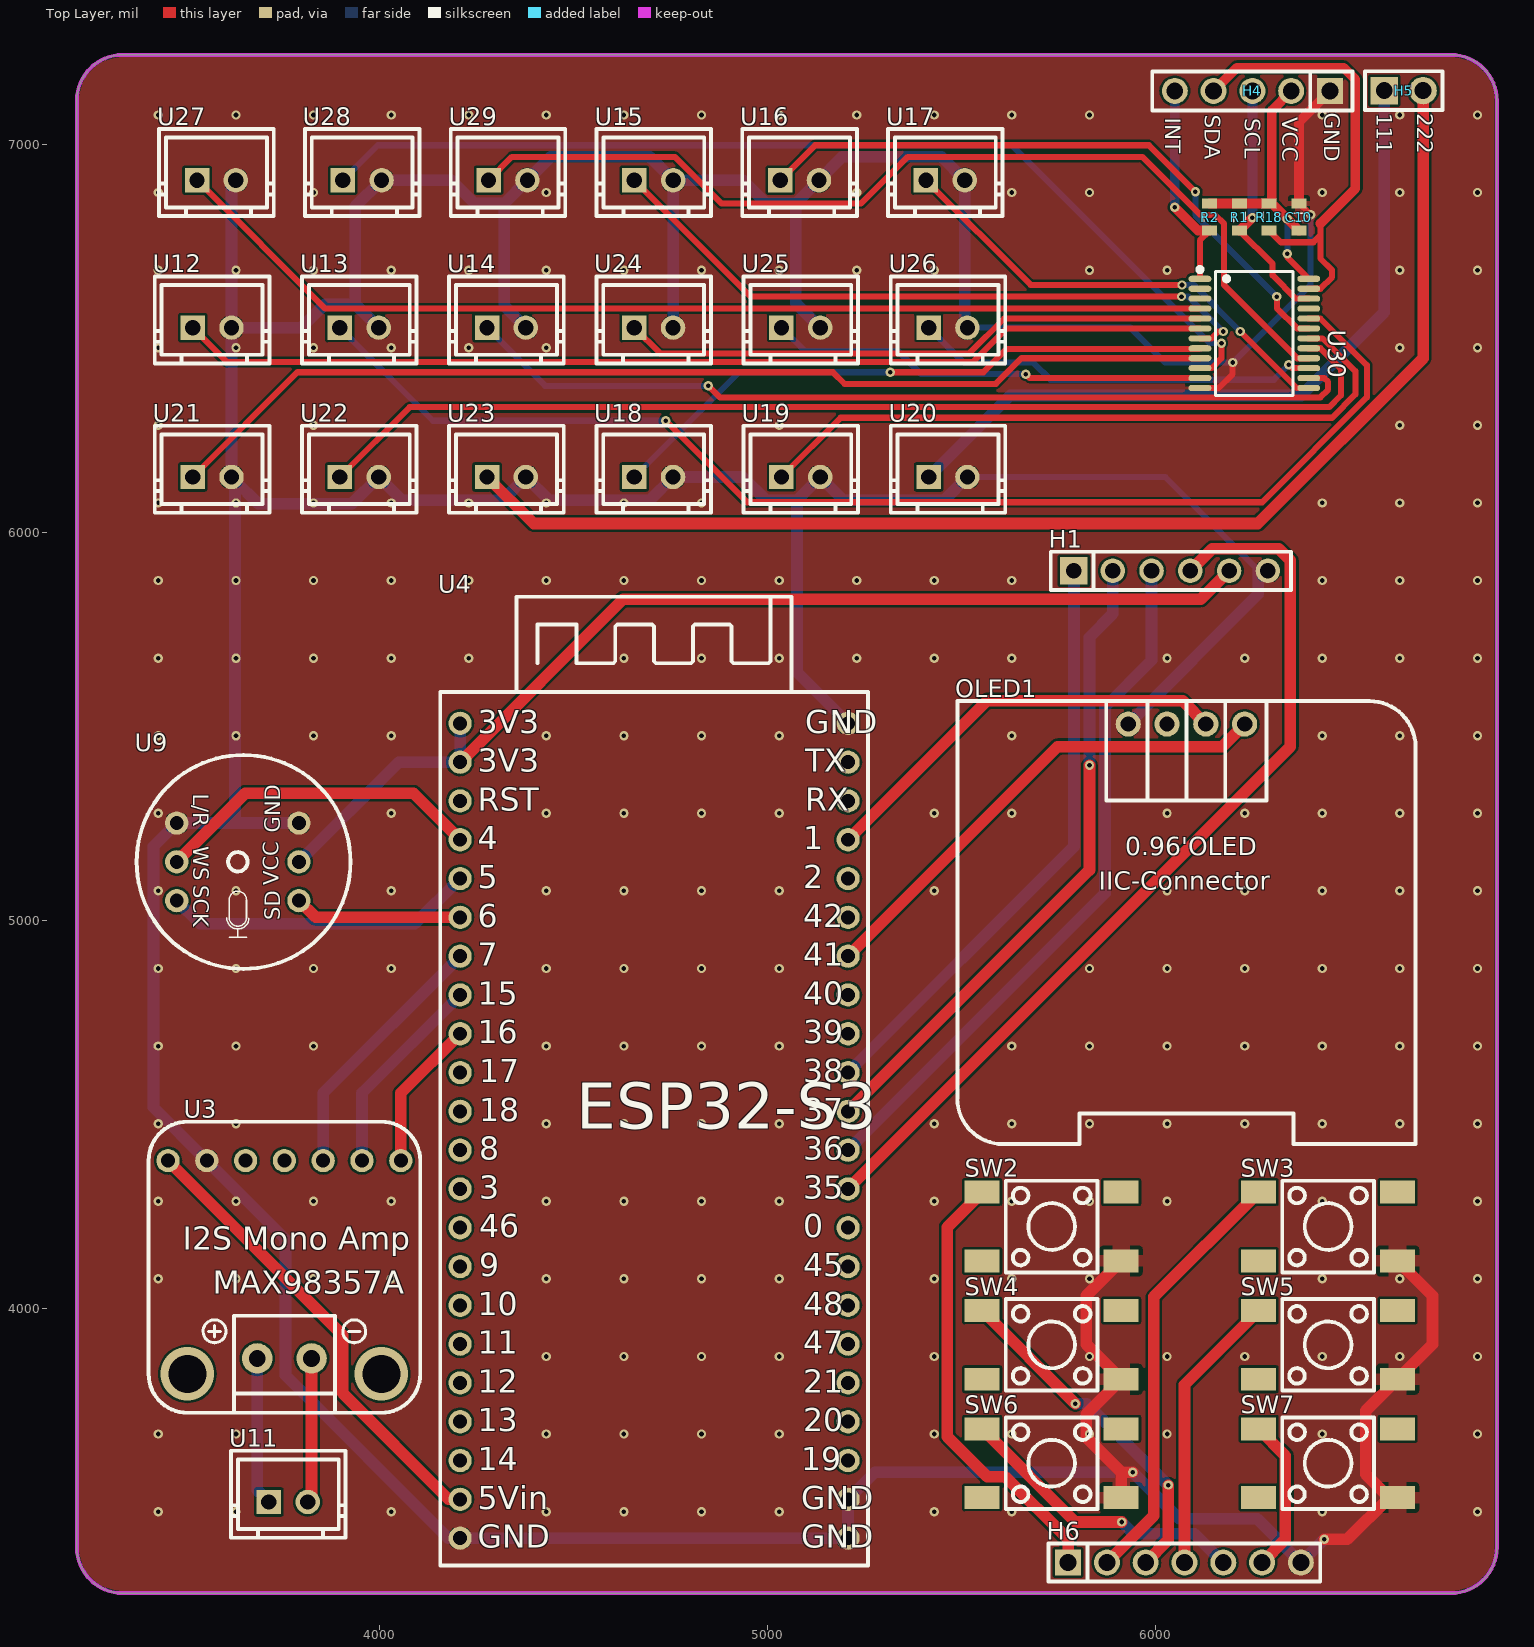
[diagram p0: Top Layer view]
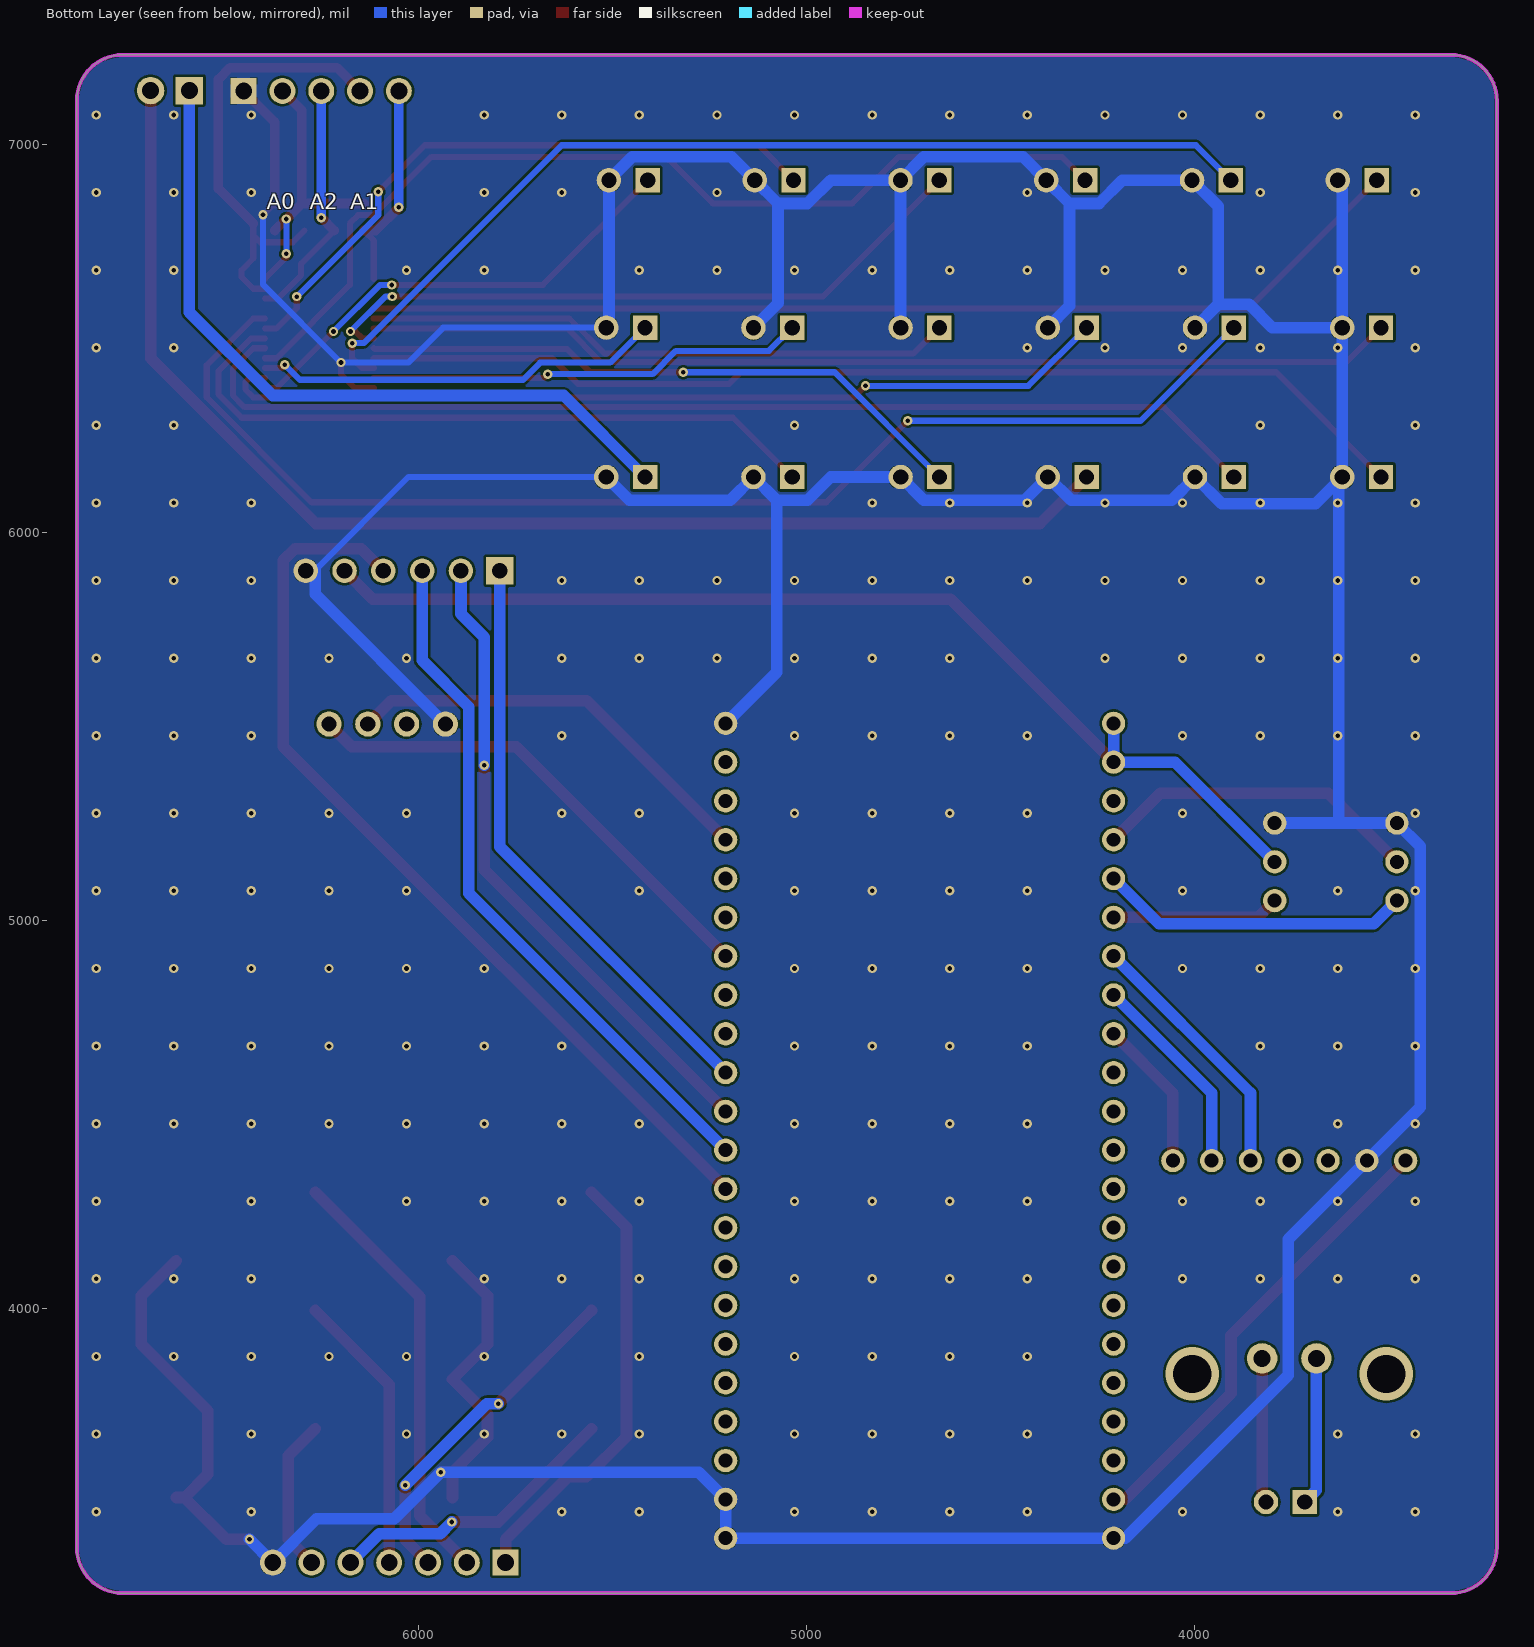
[diagram p1: Bottom Layer view, seen from below]
# Altium PCB MISC49879.pcbdoc
Units mil, origin at the board's own origin, x right, y up, seen from the top; angles counter-clockwise.
Board outline 3660 x 3965 mil, 2 copper layers (Top Layer, Bottom Layer), stack 62.206 mil thick; 38 components, 74 nets, 177 pads, 263 vias.

## Layer stack, top to bottom
Top Solder Mask Layer: solder mask 0.394, Dk 3.3
Top Layer: signal copper 1.379
Dielectric1: surface 59.449, FR4, Dk 4.5
Bottom Layer: signal copper 1.378
Bottom Solder Mask Layer: solder mask 0.394, Dk 3.3

## Board outline
3338.11,7230 ccw(c3338.11,7111.89) 3220,7111.89 3220,3383.11 ccw(c3338.11,3383.11) 3338.11,3265 6761.89,3265 ccw(c6761.89,3383.11) 6880,3383.11 6880,7111.89 ccw(c6761.89,7111.89) 6761.89,7230

## Design rules (kind name [scope] priority, off if disabled: settings)
BoardOutlineClearance Plane_Default_1 [All] p2 off: genericclearance=6 ignorepadtopadclearanceinfootprint=FALSE except(0: Arc-SplitContinuation Track-SplitContinuation SMDPad-SplitContinuation THPad-SplitContinuation Via-SplitContinuation Fill-SplitContinuation Region-SplitContinuation Poly-SplitContinuation Text-SplitContinuation Hole-SplitContinuation; 6: Arc-OutlineEdge Track-OutlineEdge SMDPad-OutlineEdge THPad-OutlineEdge Via-OutlineEdge Fill-OutlineEdge Region-OutlineEdge Poly-OutlineEdge Text-OutlineEdge Hole-OutlineEdge Arc-CutoutEdge Track-CutoutEdge SMDPad-CutoutEdge THPad-CutoutEdge Via-CutoutEdge Fill-CutoutEdge Region-CutoutEdge Poly-CutoutEdge Text-CutoutEdge Hole-CutoutEdge)
BoardOutlineClearance Copper_Default_1 [All] p4 off: genericclearance=6 ignorepadtopadclearanceinfootprint=FALSE except(0: Arc-SplitContinuation Track-SplitContinuation SMDPad-SplitContinuation THPad-SplitContinuation Via-SplitContinuation Fill-SplitContinuation Region-SplitContinuation Poly-SplitContinuation Text-SplitContinuation Hole-SplitContinuation; 6: Arc-OutlineEdge Track-OutlineEdge SMDPad-OutlineEdge THPad-OutlineEdge Via-OutlineEdge Fill-OutlineEdge Region-OutlineEdge Poly-OutlineEdge Text-OutlineEdge Hole-OutlineEdge Arc-CutoutEdge Track-CutoutEdge SMDPad-CutoutEdge THPad-CutoutEdge Via-CutoutEdge Fill-CutoutEdge Region-CutoutEdge Poly-CutoutEdge Text-CutoutEdge Hole-CutoutEdge)
BoardOutlineClearance Copper_gge24019_1 [All] p6 off: genericclearance=6 ignorepadtopadclearanceinfootprint=FALSE except(0: Arc-SplitContinuation Track-SplitContinuation SMDPad-SplitContinuation THPad-SplitContinuation Via-SplitContinuation Fill-SplitContinuation Region-SplitContinuation Poly-SplitContinuation Text-SplitContinuation Hole-SplitContinuation; 6: Arc-OutlineEdge Track-OutlineEdge SMDPad-OutlineEdge THPad-OutlineEdge Via-OutlineEdge Fill-OutlineEdge Region-OutlineEdge Text-OutlineEdge Hole-OutlineEdge Arc-CutoutEdge Track-CutoutEdge SMDPad-CutoutEdge THPad-CutoutEdge Via-CutoutEdge Fill-CutoutEdge Region-CutoutEdge Text-CutoutEdge Hole-CutoutEdge; 10: Poly-OutlineEdge Poly-CutoutEdge)
BoardOutlineClearance Default_1 [All] p8: genericclearance=6 ignorepadtopadclearanceinfootprint=FALSE except(0: Arc-SplitContinuation Track-SplitContinuation SMDPad-SplitContinuation THPad-SplitContinuation Via-SplitContinuation Fill-SplitContinuation Region-SplitContinuation Poly-SplitContinuation Text-SplitContinuation Hole-SplitContinuation; 6: Arc-OutlineEdge Track-OutlineEdge SMDPad-OutlineEdge THPad-OutlineEdge Via-OutlineEdge Fill-OutlineEdge Region-OutlineEdge Poly-OutlineEdge Text-OutlineEdge Hole-OutlineEdge Arc-CutoutEdge Track-CutoutEdge SMDPad-CutoutEdge THPad-CutoutEdge Via-CutoutEdge Fill-CutoutEdge Region-CutoutEdge Poly-CutoutEdge Text-CutoutEdge Hole-CutoutEdge)
Clearance Plane_Default [All] p1 off: gap=6 ignorepadtopadclearanceinfootprint=FALSE
Clearance Copper_Default [All] p3 off: gap=6 ignorepadtopadclearanceinfootprint=FALSE
Clearance Copper_gge24019 [All] p5 off: gap=6 ignorepadtopadclearanceinfootprint=FALSE except(10: Poly-Track Poly-SMDPad Poly-THPad Poly-Via Poly-Fill Poly-Region Poly-Poly Poly-Arc Poly-Text Poly-Hole)
Clearance Default [All] p7: gap=6 ignorepadtopadclearanceinfootprint=FALSE
DiffPairsRouting differentialPair [All] p1: maxlimit=6 minlimit=6 mostfreqgap=6 toplayer_minwidth=5 toplayer_prefwidth=10 toplayer_maxwidth=100 toplayer_mingap=6 toplayer_prefgap=6 toplayer_maxgap=6 bottomlayer_minwidth=5 bottomlayer_prefwidth=10 bottomlayer_maxwidth=100 bottomlayer_mingap=6 bottomlayer_prefgap=6 bottomlayer_maxgap=6 maxuncoupledlength=10
HoleToHoleClearance otherClearance [All] p1: gap=11.8 allowstackedmicrovias=TRUE
Length netLength [All] p1: minlimit=0 maxlimit=0
PasteMaskExpansion Common [All] p1: expansion=0
PlaneConnect Default_4 [All] p1: planeconnectstyle=Relief reliefexpansion=20 reliefentries=4 reliefconductorwidth=0 reliefairgap=10
PolygonConnect gge24019 [All] p1 off: connectstyle=Relief reliefconductorwidth=0 reliefentries=4 polygonreliefangle="90 Angle" airgapwidth=1 via.connectstyle=Relief via.reliefconductorwidth=10 via.reliefentries=4 via.polygonreliefangle="90 Angle" via.airgapwidth=10
PolygonConnect Default_5 [All] p2: connectstyle=Relief reliefconductorwidth=0 reliefentries=4 polygonreliefangle="90 Angle" airgapwidth=1 via.connectstyle=Relief via.reliefconductorwidth=10 via.reliefentries=4 via.polygonreliefangle="90 Angle" via.airgapwidth=10
RoutingVias Default_3 [All] p1: holewidth=12 width=24 viastyle="Through Hole" minholewidth=12 minwidth=24 maxholewidth=2362 maxwidth=3938
SolderMaskExpansion Common_1 [IsVia] p1: expansion=-1000 istentingtop=TRUE
SolderMaskExpansion Common_1 [All] p2: expansion=2 istentingtop=FALSE
Width Default_2 [All] p1: maxlimit=1000 minlimit=10 preferedwidth=30

## Components (designator, comment, footprint, x,y, rotation, side; value= is the part's Value field where it differs from the comment)
C10 "0.1uF" C0603-1 6370,6812 r270 top
H1 "" HDR-TH_6P-P2.54-V-F 6040,5900 r0 top
H4 "KH-2.54PH180-1X5P-L11.5" HDR-TH_5P-P2.54-V-M 6250,7137 r180 top
H5 "" HDR-TH_2P-P2.54-V-M-1 6639.9,7137.78 r0 top
H6 "" HDR-TH_7P-P2.54-V-M 6074.9,3343.84 r0 top
OLED1 "" 0.96OLED_4P 6080,5505 r0 top
R1 "4.7K" R0603-1 6216.67,6812 r90 top
R2 "4.7K" R0603-1 6140,6812 r90 top
R18 "4.7K" R0603-1 6293.33,6812 r90 top
SW2 "KH-6X6X5H-STM" SW-SMD_4P-L6.0-W6.0-P4.50-LS9.0-2 5732.51,4210 r0 top
SW3 "KH-6X6X5H-STM" SW-SMD_4P-L6.0-W6.0-P4.50-LS9.0-2 6445,4210 r0 top
SW4 "KH-6X6X5H-STM" SW-SMD_4P-L6.0-W6.0-P4.50-LS9.0-2 5732.51,3905 r0 top
SW5 "KH-6X6X5H-STM" SW-SMD_4P-L6.0-W6.0-P4.50-LS9.0-2 6445,3905 r0 top
SW6 "KH-6X6X5H-STM" SW-SMD_4P-L6.0-W6.0-P4.50-LS9.0-2 5732.51,3600 r0 top
SW7 "KH-6X6X5H-STM" SW-SMD_4P-L6.0-W6.0-P4.50-LS9.0-2 6445,3600 r0 top
U3 "Adafruit MAX98357 I2S Amp" "MAX98357 I2S AMP MODULE" 3755,4380 r270 top
U4 "NO" ESP32S3 4707.78,4461.89 r0 top
U9 "INMP441" INMP441 3635,5150 r0 top
U11 "_x001F_XH2.54-2P" CONN-TH_2P-P2.54-V 3765,3500 r0 top
U12 "_x001F_XH2.54-2P" CONN-TH_2P-P2.54-V 3568.61,6526.9 r0 top
U13 "_x001F_XH2.54-2P" CONN-TH_2P-P2.54-V 3947.98,6526.9 r0 top
U14 "_x001F_XH2.54-2P" CONN-TH_2P-P2.54-V 4327.34,6526.9 r0 top
U15 "_x001F_XH2.54-2P" CONN-TH_2P-P2.54-V 4707.04,6906.91 r0 top
U16 "_x001F_XH2.54-2P" CONN-TH_2P-P2.54-V 5082.79,6906.91 r0 top
U17 "_x001F_XH2.54-2P" CONN-TH_2P-P2.54-V 5458.54,6906.91 r0 top
U18 "_x001F_XH2.54-2P" CONN-TH_2P-P2.54-V 4706.71,6141.91 r0 top
U19 "_x001F_XH2.54-2P" CONN-TH_2P-P2.54-V 5086.07,6141.91 r0 top
U20 "_x001F_XH2.54-2P" CONN-TH_2P-P2.54-V 5465.44,6141.91 r0 top
U21 "_x001F_XH2.54-2P" CONN-TH_2P-P2.54-V 3568.61,6141.91 r0 top
U22 "_x001F_XH2.54-2P" CONN-TH_2P-P2.54-V 3947.98,6141.91 r0 top
U23 "_x001F_XH2.54-2P" CONN-TH_2P-P2.54-V 4327.34,6141.91 r0 top
U24 "_x001F_XH2.54-2P" CONN-TH_2P-P2.54-V 4706.71,6526.9 r0 top
U25 "_x001F_XH2.54-2P" CONN-TH_2P-P2.54-V 5086.07,6526.9 r0 top
U26 "_x001F_XH2.54-2P" CONN-TH_2P-P2.54-V 5465.44,6526.9 r0 top
U27 "_x001F_XH2.54-2P" CONN-TH_2P-P2.54-V 3579.8,6906.91 r0 top
U28 "_x001F_XH2.54-2P" CONN-TH_2P-P2.54-V 3955.55,6906.91 r0 top
U29 "_x001F_XH2.54-2P" CONN-TH_2P-P2.54-V 4331.3,6906.91 r0 top
U30 "PCF8575TS/1,112" SSOP-24_L8.2-W5.3-P0.65-LS7.8-BL 6255,6512 r270 top

## Footprints (in the part's own frame and the unit in brackets; to place one, negate y for a bottom-side part, rotate by r counter-clockwise, add the part's x,y. Pads: shape width x height; smd on the part's side, far side on the other; paste and mask are expansions set on the pad)
0.96OLED_4P [mm]
  round 1.65 hole 1 copper offset 0,0: 1(-3.81,-0.001) 2(-1.27,0.002) 3(1.27,0.002) 4(3.81,0.002)
  silkscreen extent -15,-27.5 15,1.5
C0603-1 [mil]
  rect 25x38.58 smd paste+0 mask+4: 1(-35,0) 2(35,0)
  silkscreen extent -10,-15 10,16
CONN-TH_2P-P2.54-V [mm]
  rect 1.6x1.6 hole 1: 1(-1.27,0)
  round 1.6 hole 1: 2(1.27,0)
  silkscreen extent -3.75,-2.34 3.75,3.36
ESP32S3 [mil]
  round 60 hole 36: 1(-500,-1055) 2(-500,-955) 3(-500,-855) 4(-500,-755) 5(-500,-655) 6(-500,-555) 7(-500,-455) 8(-500,-355) 9(-500,-255) 10(-500,-155) 11(-500,-55) 12(-500,45) 13(-500,145) 14(-500,245) 15(-500,345) 16(-500,445) 17(-500,545) 18(-500,645) 19(-500,745) 20(-500,845) 21(-500,945) 22(-500,1045) 23(500,-1055) 24(500,-955) 25(500,-855) 26(500,-755) 27(500,-655) 28(500,-555) 29(500,-455) 30(500,-355) 31(500,-255) 32(500,-155) 33(500,-55) 34(500,45) 35(500,145) 36(500,245) 37(500,345) 38(500,445) 39(500,545) 40(500,645) 41(500,745) 42(500,845) 43(500,945) 44(500,1045)
  silkscreen extent -551,-1126 551,1371
HDR-TH_2P-P2.54-V-M-1 [mm]
  rect 1.8x1.8 hole 1.1: 1(-1.27,0)
  round 1.8 hole 1.1: 2(1.27,0)
  silkscreen extent -2.54,-1.27 2.54,1.27
HDR-TH_5P-P2.54-V-M [mm]
  rect 1.7x1.7 hole 1.1: 1(-5.08,0)
  round 1.7 hole 1.1: 2(-2.54,0) 3(0,0) 4(2.54,0) 5(5.08,0)
  silkscreen extent -6.56,-1.27 6.56,1.27
HDR-TH_6P-P2.54-V-F [mm]
  rect 1.8x1.8 hole 1.02: 1(-6.35,0)
  round 1.6 hole 1.02: 2(-3.81,0) 3(-1.27,0) 4(1.27,0) 5(3.81,0) 6(6.35,0)
  silkscreen extent -7.87,-1.25 7.87,1.25
HDR-TH_7P-P2.54-V-M [mm]
  rect 1.7x1.7 hole 1.1: 1(-7.62,0)
  round 1.7 hole 1.1: 2(-5.08,0) 3(-2.54,0) 4(0,0) 5(2.54,0) 6(5.08,0) 7(7.62,0)
  silkscreen extent -8.89,-1.25 8.89,1.25
INMP441 [mil]
  round 60 hole 36: 1(157.49,100) 2(157.49,0) 3(157.49,-100) 4(-157.47,100) 5(-157.47,0) 6(-157.47,-100)
  silkscreen extent -261,-276 290,275
"MAX98357 I2S AMP MODULE" [mil]
  round 60 hole 36: 1(0,300) 2(0,200) 3(0,100) 4(0,0) 5(0,-100) 6(0,-200) 7(0,-300)
  round 78.74 hole 43.31 paste+0 mask+4: 8(510,-70) 9(510,70)
  silkscreen extent -100,-350 650,350
R0603-1 [mil]
  rect 25x38.58 smd paste+0 mask+4: 1(-35,0) 2(35,0)
  silkscreen extent -13,-15 12,15
SSOP-24_L8.2-W5.3-P0.65-LS7.8-BL [mm]
  oval 0.4x1.5 smd: 1(-3.575,-3.562) 2(-2.925,-3.562) 3(-2.275,-3.562) 4(-1.625,-3.562) 5(-0.975,-3.562) 6(-0.325,-3.562) 7(0.325,-3.562) 8(0.975,-3.562) 9(1.625,-3.562) 10(2.275,-3.562) 11(2.925,-3.562) 12(3.575,-3.562) 13(3.575,3.562) 14(2.925,3.562) 15(2.275,3.562) 16(1.625,3.562) 17(0.975,3.562) 18(0.325,3.562) 19(-0.325,3.562) 20(-0.975,3.562) 21(-1.625,3.562) 22(-2.275,3.562) 23(-2.925,3.562) 24(-3.575,3.562)
  silkscreen extent -4.33,-3.71 4.06,2.54
SW-SMD_4P-L6.0-W6.0-P4.50-LS9.0-2 [mm]
  rect 2.3x1.5 smd: 1(-4.55,2.25) 2(4.55,2.25) 3(-4.55,-2.25) 4(4.55,-2.25)
  silkscreen extent -3,-3 3,3

## Via types
v1: diameter 24, hole 12, Top Layer to Bottom Layer, 261 vias
v2: diameter 137.8, hole 98.4, Top Layer to Bottom Layer, 2 vias

## Nets (pads, with @x,y where several pads share a name; then routed paths per layer and width w, separated by ;. In a path a pad name is that pad's centre, name@x,y a point inside that pad or via, vN(x,y) a via of type N, cw(c..) or ccw(c..) an arc to the next point about the centre after c; other vN are vias at no path point)
0: U4.31
1: OLED1.3 U4.41 | length 1095.4
  Top Layer w30: U4.41 5565.94,5565.05 6070,5565.05 OLED1.3@6130,5505.05
2: U4.40
3: U4.10
3.3V: H1.5 U4.21 U4.22 U9.2 | length 2808.2
  Top Layer w30: U4.21 4627.78,5826.89 6116.89,5826.89 H1.5
  Bottom Layer w30: U9.2 4049.37,5406.89 U4.21 U4.22
4: U4.19 U9.5 | length 853.2
  Top Layer w30: U9.5 3654.41,5326.89 4087.78,5326.89 U4.19
5: U4.18 U9.6 | length 803.5
  Bottom Layer w30: U9.6 3537.52,4990 4090.89,4990 U4.18
5V-VIN: U3.7 U4.2 | length 1202.3
  Top Layer w30: U3.7 3905,3930 3905,3780 4178.11,3506.89 U4.2
6: U4.17 U9.3 | length 433.2
  Top Layer w30: U9.3 3835.59,5006.89 U4.17
7: U3.3 U4.16 | length 673
  Bottom Layer w30: U3.3 3855,4554.11 U4.16
8: U4.11
9: U4.8
10: U4.7
11: U4.6
12: U4.5
13: U4.4
14: U4.3
15: U3.2 U4.15 | length 531.6
  Bottom Layer w30: U3.2 3955,4554.11 U4.15
16: U3.1 U4.14 | length 390.2
  Top Layer w30: U3.1 4055,4554.11 U4.14
17: U4.13
18: U4.12
19: U4.25
20: U4.26
21: U4.27
35: H1.4 U4.32 | length 2386
  Top Layer w30: U4.32 6347.78,5446.89 6347.78,5926.89 6317.78,5956.89 6146.89,5956.89 H1.4
36: H1.3 U4.33 | length 1817.1
  Bottom Layer w30: U4.33 5870,5069.11 5870,5549.11 5990,5669.11 H1.3
37: H1.2 U4.34 | length 1675.7
  Top Layer w30: U4.34 5830,5129.11 v1(5830,5399.11)
  Bottom Layer w30: v1(5830,5399.11) 5830,5729.11 5890,5789.11 H1.2
38: H1.1 U4.35 | length 1534.3
  Bottom Layer w30: U4.35 5790,5189.11 H1.1
39: U4.36
40: U4.37
41: OLED1.4 U4.38 | length 1270
  Top Layer w30: U4.38 5747.78,5446.89 6171.84,5446.89 OLED1.4@6230,5505.05
42: U4.39
45: U4.30
46: U4.9
47: U4.28
48: U4.29
111: H5.1 U20.1 | length 1921.7
  Bottom Layer w30: U20.1 5625.44,6351.91 6375.44,6351.91 6589.9,6566.37 H5.1
222: H5.2 U23.1 | length 3328.7
  Top Layer w30: U23.1 4397.34,6021.91 6264.03,6021.91 6689.9,6447.78 H5.2
$1N6791: H6.1 SW2.1 | length 1148.5
  Top Layer w30: SW2.1 5463.38,4208.59 5463.38,3668.59 5566.6,3565.36 5613.38,3565.36 5774.9,3403.84 H6.1
$1N6796: H6.2 SW3.1 | length 1116.7
  Top Layer w30: H6.2 5995.87,3464.81 5995.87,4028.59 SW3.1
$1N6804: H6.3 SW4.1 | length 890.4
  Top Layer w30: SW4.1 v1(5793.38,3753.59) ; H6.3 6033.38,3402.32 v1(6033.38,3543.59)
  Bottom Layer w30: v1(5793.38,3753.59) 5823.38,3753.59 v1(6033.38,3543.59)
$1N6814: H6.4 SW5.1 | length 728.8
  Top Layer w30: H6.4 6074.9,3802.61 SW5.1
$1N6821: H6.5 SW6.1 | length 764.3
  Top Layer w30: SW6.1 5793.38,3448.59 v1(5913.38,3448.59)
  Bottom Layer w30: v1(5913.38,3448.59) 5943.38,3418.59 6100.15,3418.59 H6.5
$1N6831: H6.6 SW7.1 | length 398.2
  Top Layer w30: SW7.1 6334.9,3619.56 6334.9,3403.84 H6.6
+5V: OLED1.2
A0: U30.21
A1: U30.2
A2: U30.3
GND: C10.1 H1.6 H4.1 H6.7 OLED1.1 SW2.4 SW3.4 SW4.4 SW5.4 SW6.4 SW7.4 U3.6 U4.1 U4.23 U4.24 U4.44 U9.1 U9.4 U12.2 U13.2 U14.2 U15.2 U16.2 U17.2 U18.2 U19.2 U20.2 U21.2 U22.2 U23.2 U24.2 U25.2 U26.2 U27.2 U28.2 U29.2 U30.12 | length 18226.5
  Top Layer w15.75: U30.12 6163.46,6371.25 6199.11,6406.9 v1(6199.11,6436.9) ; C10.1 v1(6400,6817.79)
  Top Layer w25: C10.1 6370,7057 H4.1
  Top Layer w30: SW6.4 5911.64,3576.41 ; SW2.4 5821.64,4031.41 5821.64,3906.41 SW4.4 5821.64,3726.41 5821.64,3666.41 5911.64,3576.41 ; v1(5941.64,3576.41) 5911.64,3576.41 ; v1(6434.9,3403.84) 6494.9,3403.84 SW7.4@6602.48,3511.41 ; SW7.4 SW7.4@6602.48,3511.41 ; SW3.4 6714.13,4031.41 6714.13,3906.41 SW5.4 6542.48,3734.76 6542.48,3571.41 SW7.4@6602.48,3511.41
  Bottom Layer w15.75: U20.2 6025.44,6141.91 6265.44,5901.91 H1.6 ; U26.2 5935.44,6526.9 6025.44,6436.9 v1(6199.11,6436.9) 6400,6637.79 v1(6400,6817.79)
  Bottom Layer w30: U27.2 3618.61,6895.72 U12.2 ; U9.1 3627.52,5250 ; U13.2 3937.98,6586.9 ; U14.2 4321.3,6582.94 4321.3,6846.91 ; U24.2 4757.04,6527.24 U15.2 ; U25.2 5072.79,6590.18 5072.79,6846.91 ; U4.44 5076.07,5638.6 5076.07,6081.91 ; U20.2 5455.44,6081.91 5196.07,6081.91 U19.2 5076.07,6081.91 ; U26.2 5508.54,6533.8 U17.2 5448.54,6966.91 5192.79,6966.91 U16.2 5072.79,6846.91 ; OLED1.1 6265.44,5840.39 H1.6@6265.44,5901.91 ; v1(6434.9,3403.84) H6.7 6262.32,3456.41 6061.64,3456.41 v1(5941.64,3576.41) 5277.3,3576.41 U4.24 U4.23 U4.1 4177.78,3406.89 3757.78,3826.89 3757.78,4177.22 U3.6 3417.52,4517.48 3417.52,5190 U9.4 3627.52,5250 ; U12.2 U21.2 U21.2@3627.52,6133 ; U12.2 3798.61,6526.9 3858.61,6586.9 3937.98,6586.9 ; 3627.52,5250 U21.2@3627.52,6133 ; U21.2@3627.52,6133 3687.52,6073 3929.07,6073 U22.2 4057.98,6081.91 4317.34,6081.91 U23.2 4437.34,6081.91 4696.71,6081.91 U18.2 4936.71,6141.91 4996.71,6081.91 5076.07,6081.91 ; 3937.98,6586.9 3937.98,6839.33 U28.2 4185.55,6906.91 4245.55,6846.91 4321.3,6846.91 ; 4321.3,6846.91 U29.2 4441.3,6966.91 4697.04,6966.91 U15.2 ; U15.2 4937.04,6906.91 4997.04,6846.91 5072.79,6846.91
  other v1: 3430.1,3475.1 3630.1,3475.1 4030.1,3475.1 4430.1,3475.1 4630.1,3475.1 4830.1,3475.1 5030.1,3475.1 5430.1,3475.1 5630.1,3475.1 6430.1,3475.1 6830.1,3475.1 3430.1,3675.1 3630.1,3675.1 4430.1,3675.1 4630.1,3675.1 4830.1,3675.1 5030.1,3675.1 5430.1,3675.1 5630.1,3675.1 5830.1,3675.1 6030.1,3675.1 6430.1,3675.1 6830.1,3675.1 4430.1,3875.1 4630.1,3875.1 4830.1,3875.1 5030.1,3875.1 5430.1,3875.1 5830.1,3875.1 6030.1,3875.1 6230.1,3875.1 6430.1,3875.1 6630.1,3875.1 6830.1,3875.1 3430.1,4075.1 3630.1,4075.1 3830.1,4075.1 4030.1,4075.1 4430.1,4075.1 4630.1,4075.1 4830.1,4075.1 5030.1,4075.1 5430.1,4075.1 5630.1,4075.1 5830.1,4075.1 6430.1,4075.1 6630.1,4075.1 6830.1,4075.1 3430.1,4275.1 3630.1,4275.1 3830.1,4275.1 4030.1,4275.1 4430.1,4275.1 4630.1,4275.1 4830.1,4275.1 5030.1,4275.1 5430.1,4275.1 5630.1,4275.1 5830.1,4275.1 6030.1,4275.1 6430.1,4275.1 6830.1,4275.1 3430.1,4475.1 3630.1,4475.1 4430.1,4475.1 4630.1,4475.1 4830.1,4475.1 5030.1,4475.1 5430.1,4475.1 5630.1,4475.1 5830.1,4475.1 6030.1,4475.1 6230.1,4475.1 6430.1,4475.1 6630.1,4475.1 6830.1,4475.1 3430.1,4675.1 3630.1,4675.1 3830.1,4675.1 4430.1,4675.1 4630.1,4675.1 4830.1,4675.1 5030.1,4675.1 5630.1,4675.1 5830.1,4675.1 6030.1,4675.1 6230.1,4675.1 6430.1,4675.1 6630.1,4675.1 6830.1,4675.1 3430.1,4875.1 3630.1,4875.1 3830.1,4875.1 4030.1,4875.1 4430.1,4875.1 4630.1,4875.1 4830.1,4875.1 5030.1,4875.1 5830.1,4875.1 6030.1,4875.1 6230.1,4875.1 6430.1,4875.1 6630.1,4875.1 6830.1,4875.1 3430.1,5075.1 3630.1,5075.1 4030.1,5075.1 4430.1,5075.1 4630.1,5075.1 4830.1,5075.1 5030.1,5075.1 5430.1,5075.1 6030.1,5075.1 6230.1,5075.1 6430.1,5075.1 6630.1,5075.1 6830.1,5075.1 3430.1,5275.1 4030.1,5275.1 4430.1,5275.1 4630.1,5275.1 4830.1,5275.1 5030.1,5275.1 5430.1,5275.1 5630.1,5275.1 6030.1,5275.1 6230.1,5275.1 6430.1,5275.1 6630.1,5275.1 6830.1,5275.1 3430.1,5475.1 3630.1,5475.1 3830.1,5475.1 4030.1,5475.1 4430.1,5475.1 4630.1,5475.1 4830.1,5475.1 5030.1,5475.1 5630.1,5475.1 6430.1,5475.1 6630.1,5475.1 6830.1,5475.1 3430.1,5675.1 3630.1,5675.1 3830.1,5675.1 4030.1,5675.1 4230.1,5675.1 4630.1,5675.1 4830.1,5675.1 5030.1,5675.1 5230.1,5675.1 5430.1,5675.1 5630.1,5675.1 6030.1,5675.1 6230.1,5675.1 6430.1,5675.1 6630.1,5675.1 6830.1,5675.1 3430.1,5875.1 3630.1,5875.1 3830.1,5875.1 4030.1,5875.1 4230.1,5875.1 4430.1,5875.1 4630.1,5875.1 4830.1,5875.1 5030.1,5875.1 5230.1,5875.1 5430.1,5875.1 5630.1,5875.1 6430.1,5875.1 6630.1,5875.1 6830.1,5875.1 3430.1,6075.1 3630.1,6075.1 3830.1,6075.1 4030.1,6075.1 4230.1,6075.1 4430.1,6075.1 4630.1,6075.1 4830.1,6075.1 6430.1,6075.1 6630.1,6075.1 6830.1,6075.1 3430.1,6275.1 3830.1,6275.1 5030.1,6275.1 6630.1,6275.1 6830.1,6275.1 3430.1,6475.1 3630.1,6475.1 3830.1,6475.1 4030.1,6475.1 4230.1,6475.1 4430.1,6475.1 6630.1,6475.1 6830.1,6475.1 3430.1,6675.1 3630.1,6675.1 3830.1,6675.1 4030.1,6675.1 4230.1,6675.1 4430.1,6675.1 4630.1,6675.1 4830.1,6675.1 5030.1,6675.1 5230.1,6675.1 5430.1,6675.1 5830.1,6675.1 6030.1,6675.1 6630.1,6675.1 6830.1,6675.1 3430.1,6875.1 3830.1,6875.1 4430.1,6875.1 5230.1,6875.1 5630.1,6875.1 5830.1,6875.1 6430.1,6875.1 6630.1,6875.1 6830.1,6875.1 3430.1,7075.1 3630.1,7075.1 3830.1,7075.1 4030.1,7075.1 4230.1,7075.1 4430.1,7075.1 4630.1,7075.1 4830.1,7075.1 5030.1,7075.1 5230.1,7075.1 5430.1,7075.1 5630.1,7075.1 5830.1,7075.1 6430.1,7075.1 6630.1,7075.1 6830.1,7075.1
INT: H4.5 R2.1 U30.1 | length 549.6
  Top Layer w15.75: U30.1 6114.76,6751.76 R2.1
  Top Layer w25: v1(6050,6837) 6110,6777 R2.1
  Bottom Layer w25: v1(6050,6837) H4.5
P00: U27.1 U30.4 | length 2722
  Top Layer w15.75: U27.1 3860.73,6575.98 U30.4
P01: U24.1 U30.5 | length 1522.9
  Top Layer w15.75: U24.1 4723.22,6460.39 5520.2,6460.39 5610.2,6550.39 U30.5
P02: U12.1 U30.6 | length 2669.1
  Top Layer w15.75: U12.1 3607.72,6437.79 5529.5,6437.79 5616.5,6524.79 U30.6
P03: U15.1 U30.7 | length 1746.6
  Top Layer w15.75: U15.1 4957.04,6606.91 v1(6067.04,6606.91) ; U30.7 6144.76,6499.2 6162.47,6516.91 v1(6174.76,6516.91)
  Bottom Layer w15.75: v1(6067.04,6606.91) 6084.76,6606.91 v1(6174.76,6516.91)
P04: U18.1 U30.8 | length 1595.4
  Top Layer w15.75: v1(5316.71,6411.91) 5556.71,6411.91 5616.71,6471.91 6113.06,6471.91 U30.8
  Bottom Layer w15.75: U18.1 4926.71,6411.91 v1(5316.71,6411.91)
P05: U21.1 U30.9 | length 2747.8
  Top Layer w15.75: U21.1 3788.61,6411.91 5168.61,6411.91 5198.61,6381.91 5588.61,6381.91 5654.72,6448.02 U30.9
P06: U28.1 U30.10 | length 2618.3
  Top Layer w15.75: U30.10 6144.76,6422.43 6170.28,6447.95 v1(6170.28,6486.91)
  Bottom Layer w15.75: U28.1 3995.55,6996.91 5630.28,6996.91 6140.28,6486.91 v1(6170.28,6486.91)
P07: U25.1 U30.11 | length 1132.6
  Top Layer w15.75: v1(5666.07,6406.9) 5676.13,6396.84 U30.11
  Bottom Layer w15.75: U25.1 5096.07,6466.9 5336.07,6466.9 5396.07,6406.9 v1(5666.07,6406.9)
P08: U17.1 U30.13 | length 1208.6
  Top Layer w15.75: U17.1 5678.54,6636.91 v1(6068.54,6636.91) ; v1(6218.54,6516.91) 6364.2,6371.25 U30.13
  Bottom Layer w15.75: v1(6068.54,6636.91) 6098.54,6636.91 v1(6218.54,6516.91)
P09: U14.1 U30.14 | length 2324.9
  Top Layer w15.75: v1(4847.34,6376.9) 4877.34,6346.9 6425.24,6346.9 6445.27,6366.93 6445.27,6386.87 6435.3,6396.84 U30.14
  Bottom Layer w15.75: U14.1 4427.34,6376.9 v1(4847.34,6376.9)
P10: U26.1 U30.15 | length 1055.1
  Top Layer w15.75: v1(6343.91,6431.1) 6352.59,6422.43 U30.15
  Bottom Layer w15.75: U26.1 5505.44,6436.9 5685.44,6436.9 5729.91,6392.43 6305.24,6392.43 v1(6343.91,6431.1)
P11: U29.1 U30.16 | length 2546
  Top Layer w15.75: U29.1 4341.3,6966.91 4761.3,6966.91 4881.3,6846.91 5241.3,6846.91 5361.3,6966.91 5966.35,6966.91 6116.35,6816.91 6154.84,6816.91 6176.35,6795.4 6176.35,6636.91 6365.24,6448.02 U30.16
P12: U22.1 U30.17 | length 2840.5
  Top Layer w15.75: U22.1 4077.98,6321.91 6447.98,6321.91 6477.98,6351.91 6477.98,6420.87 6425.24,6473.61 U30.17
P13: U19.1 U30.18 | length 1782.3
  Top Layer w15.75: U19.1 5188.78,6294.62 6455.24,6294.62 6515.24,6354.62 6515.24,6414.62 6430.66,6499.2 U30.18
P14: U16.1 U30.19 | length 1648
  Top Layer w15.75: U16.1 5122.79,6996.91 5983.12,6996.91 v1(6103.12,6876.91) ; v1(6313.12,6606.91) 6313.12,6576.91 6365.24,6524.79 U30.19
  Bottom Layer w15.75: v1(6103.12,6876.91) 6103.12,6816.91 v1(6313.12,6606.91)
P15: U13.1 U30.20 | length 3228.7
  Top Layer w15.75: v1(4737.98,6286.9) 4947.98,6076.9 6275.24,6076.9 6545.24,6346.9 6545.24,6430.39 6425.24,6550.39 U30.20
  Bottom Layer w15.75: U13.1 4137.98,6286.9 v1(4737.98,6286.9)
RST: U4.20
RX: U4.42
SCL: H4.3 R1.1 U30.22 | length 642.6
  Top Layer w15.75: R1.1 6302.1,6691.57 6302.1,6661.57 6362.1,6601.57 U30.22
  Top Layer w25: R1.1 v1(6250,6810.33)
  Bottom Layer w25: v1(6250,6810.33) H4.3
SDA: H4.4 R18.1 U30.23 | length 1186.3
  Top Layer w15.75: R18.1 6323.33,6747 6407.15,6747 6425.24,6765.09 ; U30.23 6425.24,6627.16 6455.24,6657.16 6455.24,6675.09 6425.24,6705.09 6425.24,6765.09 ; 6425.24,6795.09 6425.24,6765.09
  Top Layer w25: H4.4 6210,7197 6485.24,7197 6515.24,7167 6515.24,6885.09 6425.24,6795.09
SPEAKER+: U3.8 U11.1 | length 382.4
  Bottom Layer w30: U3.8 3685,3530 U11.1
SPEAKER-: U3.9 U11.2 | length 374.1
  Top Layer w30: U11.2 3825,3510 U3.9
TX: U4.43
VCC: C10.2 H4.2 R1.2 R2.2 R18.2 U30.24 | length 746.8
  Top Layer w15.75: v1(6340,6717) 6340,6707.99 U30.24
  Top Layer w25: R2.2 R1.2 R18.2 R18.2@6300,6847 ; H4.2 6300,7087 R18.2@6300,6847 ; C10.2 v1(6340,6807) R18.2@6300,6847
  Bottom Layer w15.75: v1(6340,6717) v1(6340,6807)
pads on no net: SW2.2 SW2.3 SW3.2 SW3.3 SW4.2 SW4.3 SW5.2 SW5.3 SW6.2 SW6.3 SW7.2 SW7.3 U3.4 U3.5
copper on no net:
  other v2: 3505,3830 4005,3830

## Polygon pours and split planes (outlines as drawn)
GND on Top Layer (solid, remove dead copper, pour order 0): 3085,7495 3085,3125 7020,3125 7020,7495
GND on Bottom Layer (solid, remove dead copper, pour order 2): 3000,7480 3000,3000 7120,3000 7120,7480

## Keep-outs
Board Outline Layer:
  the board outline again, w10

## Silkscreen, mask and mechanical layers (free items; w line width, h text height)
Top Silkscreen Layer:
  text "GND" at 6435,7081.3 h40 r270
  text "111" at 6570,7079.25 h40 r270
  text "222" at 6675,7079.25 h40 r270
  text "SDA" at 6126.97,7075.3 h40 r270
  text "VCC" at 6327.02,7069.6 h40 r270
  text "INT" at 6025,7067.95 h40 r270
  text "SCL" at 6229.73,7066.88 h40 r270
Bottom Silkscreen Layer:
  text "A1" at 6175,6831.75 h40
  text "A2" at 6280,6831.7 h40
  text "A0" at 6390,6832 h40